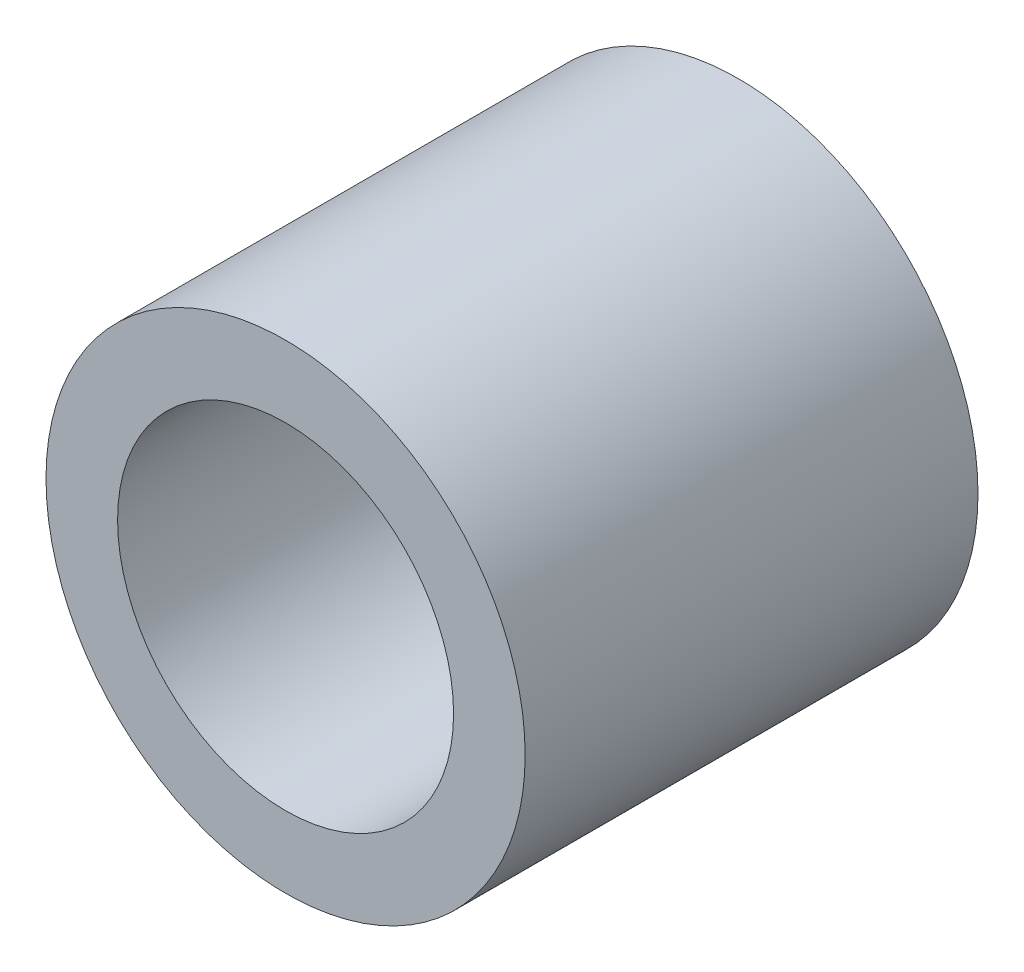
from build123d import *

# Parameters (mm, degrees)
SKETCH_1_R      = 1.64
SKETCH_1_R_2    = 1.15
EXTRUDE_1_DEPTH = 3.1


with BuildPart() as part:
    # 草图1 → 凸台-拉伸1 (new body)
    with BuildSketch(Plane.XY):
        with Locations(Location((0, 0, 0), (0, 0, 180))):
            Circle(SKETCH_1_R)
        with Locations(Location((0, 0, 0), (0, 0, 180))):
            Circle(SKETCH_1_R_2, mode=Mode.SUBTRACT)
    extrude(amount=EXTRUDE_1_DEPTH)


solid = part.part
